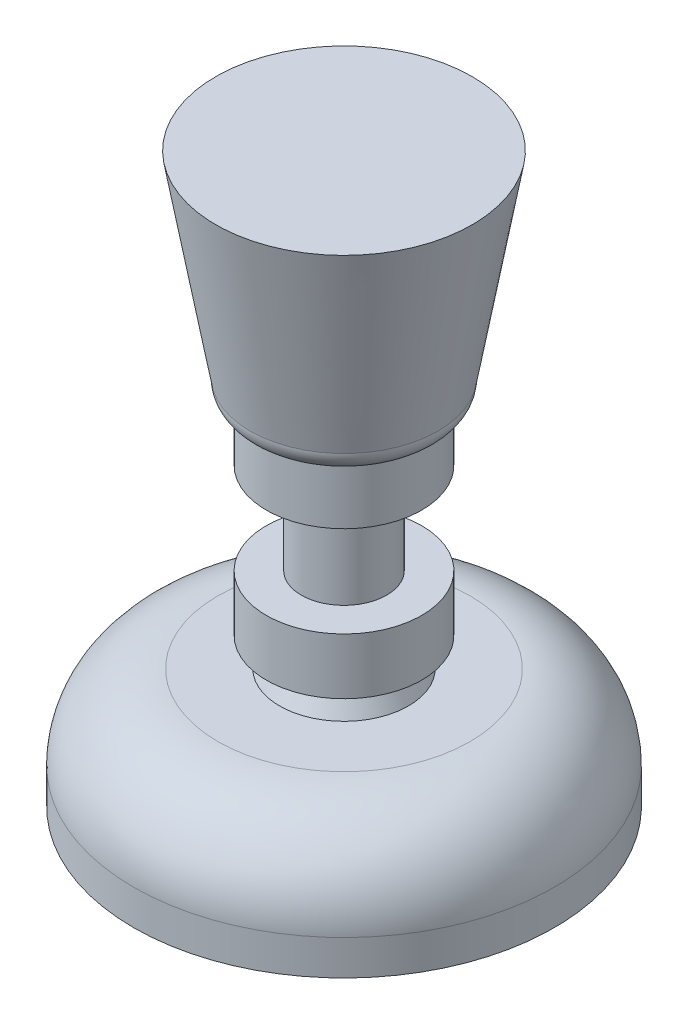
from build123d import *


with BuildPart() as part:
    # 草图1 → 旋转1 (revolve)
    with BuildSketch(Plane.XY, mode=Mode.PRIVATE) as revolve_1_sk:
        with BuildLine():
            Line((0, -19.516129032), (24, -19.516129032))
            Line((24, -19.516129032), (24, -16.516129032))
            Line((24, -16.516129032), (30, -16.516129032))
            Line((30, -16.516129032), (30, -11.516129032))
            ThreePointArc((30, -11.516129032), (26.485281374, -3.030847658), (18, 0.483870968))
            Line((18, 0.483870968), (9.2, 0.483870968))
            Line((9.2, 0.483870968), (8.089553055, 2.611524037))
            Line((8.089553055, 2.611524037), (8.089553055, 4.611524037))
            Line((8.089553055, 4.611524037), (11.089553055, 4.611524037))
            Line((11.089553055, 4.611524037), (11.089553055, 12.611524037))
            Line((11.089553055, 12.611524037), (6.089553055, 12.611524037))
            Line((6.089553055, 12.611524037), (6.089553055, 25.611524037))
            Line((6.089553055, 25.611524037), (11.089553055, 25.611524037))
            Line((11.089553055, 25.611524037), (11.089553055, 33.611524037))
            ThreePointArc((11.089553055, 33.611524037), (12.752211126, 34.669644876), (13.399553055, 36.531095923))
            Line((13.399553055, 36.531095923), (18.3, 64.483870968))
            Line((18.3, 64.483870968), (0, 64.483870968))
            Line((0, 64.483870968), (0, -19.516129032))
        make_face()
    revolve(revolve_1_sk.sketch.rotate(Axis((0, 0, 0), (0, 1, 0)), 90), axis=Axis((0, 0, 0), (0, 1, 0)))


solid = part.part
